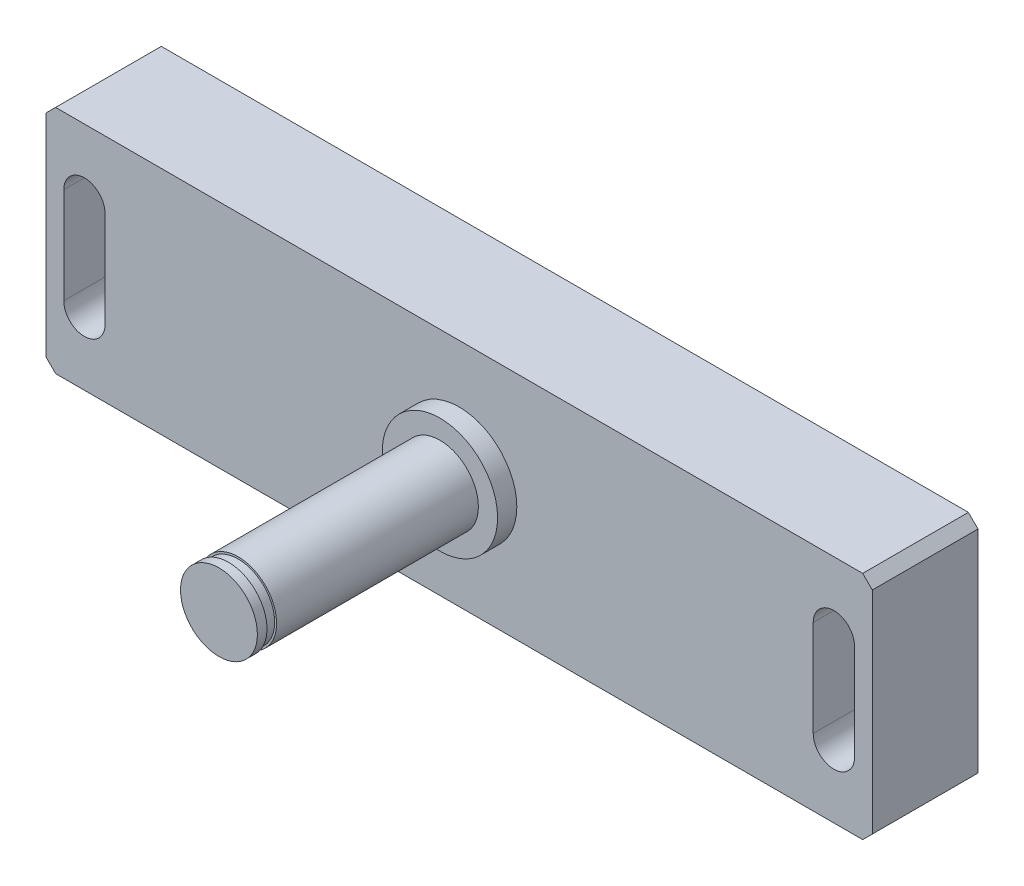
SolidWorks part; units mm, degrees
material "普通碳钢"
ref_plane "前视基准面" through (0, 0, 0) normal (0, 0, 1) x (1, 0, 0)
ref_plane "上视基准面" through (0, 0, 0) normal (0, 1, 0) x (1, 0, 0)
ref_plane "右视基准面" through (0, 0, 0) normal (1, 0, 0) x (0, 0, -1)
sketch "草图1" plane through (0, 0, 0) normal (0, 0, 1) x (1, 0, 0)
  line L1 (-43, 12) -> (43, 12)
  line L2 (-43, 12) -> (-43, -12)
  line L3 (-43, -12) -> (43, -12)
  line L4 (43, 12) -> (43, -12)
  line L5 (-43, 12) -> (43, -12) construction
  line L6 (-43, -12) -> (43, 12) construction
  point P0 (0, 0)
  dimension "D1" = 24
  dimension "D2" = 86
extrude "凸台-拉伸1" add sketch "草图1" along normal mid plane 11
sketch "草图2" plane through (0, 0, 5.5) normal (0, 0, 1) x (1, 0, 0)
  circle A0 centre (0, 0) radius 4
  dimension "D1" = 8
extrude "凸台-拉伸2" add sketch "草图2" along normal blind 3.5
sketch "草图3" plane through (0, 0, 9) normal (0, 0, 1) x (1, 0, 0)
  circle A0 centre (0, 0) radius 4
  dimension "D1" = 8
extrude "凸台-拉伸3" add sketch "草图3" along normal blind 21.5
sketch "草图4" plane through (0, 0, 0) normal (0, 1, 0) x (1, 0, 0)
  line L1 (43, -5.5) -> (-43, -5.5) construction
  line L7 (0, 0) -> (0, -30.5) construction
  line L8 (-4, -30.5) -> (4, -30.5) construction
  line L10 (-4, -5.5) -> (-4, -30.5) construction
  line L11 (-4, -28.5) -> (-3.8, -28.5)
  line L12 (-4, -28.5) -> (-4, -29.5)
  line L13 (-4, -29.5) -> (-3.8, -29.5)
  line L14 (-3.8, -28.5) -> (-3.8, -29.5)
  dimension "D1" = 0.2
  dimension "D2" = 1
  dimension "D3" = 23
sketch "草图14" plane through (0, 0, -5.5) normal (0, 0, -1) x (-1, 0, 0)
  line L0 (-39, 5) -> (-39, -5) construction
  line L1 (-36.85, 5) -> (-36.85, -5)
  line L2 (-41.15, 5) -> (-41.15, -5)
  line L3 (0, 0) -> (-43, 0) construction
  line L4 (-43, -12) -> (-43, 12) construction
  line L5 (0, 12) -> (0, -12) construction
  line L6 (-43, 12) -> (43, 12) construction
  line L7 (43, -12) -> (-43, -12) construction
  line L8 (39, 5) -> (39, -5) construction
  line L9 (36.85, 5) -> (36.85, -5)
  line L10 (41.15, 5) -> (41.15, -5)
  arc A0 (-36.85, 5) -> (-41.15, 5) centre (-39, 5) ccw
  arc A1 (-41.15, -5) -> (-36.85, -5) centre (-39, -5) ccw
  arc A2 (36.85, 5) -> (41.15, 5) centre (39, 5) cw
  arc A3 (41.15, -5) -> (36.85, -5) centre (39, -5) cw
  point P2 (-39, 0)
  point P20 (39, 0)
  dimension "D2" = 2.15
  dimension "D1" = 78
  dimension "D3" = 10
extrude "切除-拉伸4" cut sketch "草图14" against normal through all
sketch "草图15" plane through (0, 0, -5.5) normal (0, 0, -1) x (-1, 0, 0)
  circle A0 centre (0, 0) radius 4
  dimension "D1" = 8
extrude "切除-拉伸5" cut sketch "草图15" against normal blind 9.999
revolve "切除-旋转1" cut sketch "草图4" angle 360 about L7
sketch "草图16" plane through (0, 0, 4.499) normal (0, 0, -1) x (-1, 0, 0)
  circle A0 centre (0, 0) radius 2.9995
  dimension "D1" = 5.999
extrude "凸台-拉伸4" add sketch "草图16" along normal blind 8.999
sketch "草图18" plane through (0, 0, 5.5) normal (0, 0, 1) x (1, 0, 0)
  circle A0 centre (0, 0) radius 6
  dimension "D1" = 12
extrude "凸台-拉伸5" add sketch "草图18" along normal blind 2
sketch "草图22" plane through (0, 0, -5.5) normal (0, 0, -1) x (-1, 0, 0)
  circle A0 centre (0, 0) radius 7.5
  dimension "D1" = 15
extrude "凸台-拉伸7" add sketch "草图22" against normal up to surface (11 mm away) up to face at (0, 0, 5.5)
chamfer "倒角1" distance 1 angle 45 4 edges at (43, 12, 0) (-43, 12, 0) (-43, -12, 0) (43, -12, 0)
